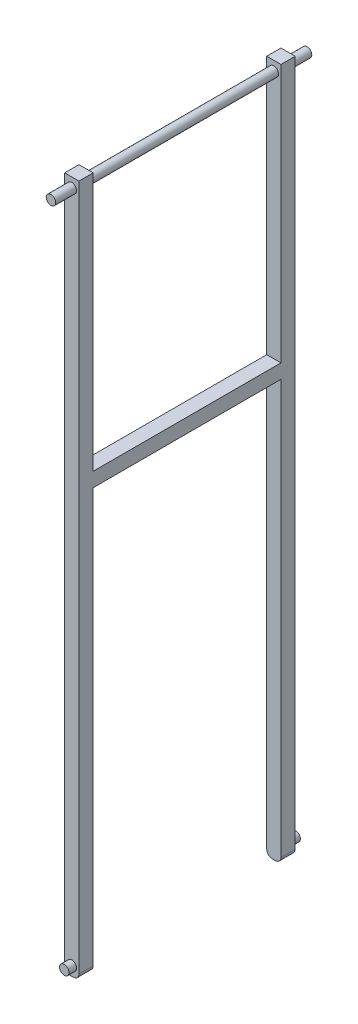
SolidWorks part; units mm, degrees
ref_plane "Front Plane" through (0, 0, 0) normal (0, 0, 1) x (1, 0, 0)
ref_plane "Top Plane" through (0, 0, 0) normal (0, 1, 0) x (1, 0, 0)
ref_plane "Right Plane" through (0, 0, 0) normal (1, 0, 0) x (0, 0, -1)
other "Configuration Table"
sketch "Sketch1" plane through (0, 0, 0) normal (0, 1, 0) x (1, 0, 0)
  line L1 (-7.5, 7.5) -> (7.5, 7.5)
  line L2 (-7.5, 7.5) -> (-7.5, -7.5)
  line L3 (-7.5, -7.5) -> (7.5, -7.5)
  line L4 (7.5, 7.5) -> (7.5, -7.5)
  line L5 (-7.5, 7.5) -> (7.5, -7.5) construction
  line L6 (-7.5, -7.5) -> (7.5, 7.5) construction
  point P0 (0, 0)
  dimension "D1" = 15
  dimension "D2" = 15
extrude "Boss-Extrude1" add sketch "Sketch1" along normal blind 730
sketch "Sketch2" plane through (0, 0, -7.5) normal (0, 0, -1) x (-1, 0, 0)
  circle A0 centre (0, 10) radius 5
  dimension "D1" = 10
  dimension "D2" = 10
extrude "Boss-Extrude2" add sketch "Sketch2" along normal blind 8
sketch "Sketch4" plane through (0, 0, 7.5) normal (0, 0, 1) x (1, 0, 0)
  line L0 (7.5, 730) -> (7.5, 0) construction
  line L1 (-7.5, 457.5) -> (7.5, 457.5)
  line L2 (-7.5, 457.5) -> (-7.5, 442.5)
  line L3 (-7.5, 442.5) -> (7.5, 442.5)
  line L4 (7.5, 457.5) -> (7.5, 442.5)
  line L5 (-7.5, 457.5) -> (7.5, 442.5) construction
  line L6 (-7.5, 442.5) -> (7.5, 457.5) construction
  line L7 (-7.5, 730) -> (7.5, 730) construction
  point P0 (0, 450)
  dimension "D1" = 15
  dimension "D2" = 15
  dimension "D3" = 450
  dimension "D4" = 280
extrude "Boss-Extrude3" add sketch "Sketch4" along normal blind 198
sketch "Sketch5" plane through (0, 0, 205.5) normal (0, 0, 1) x (1, 0, 0)
  line L0 (-7.5, 730) -> (-7.5, 457.5) construction
  line L1 (-7.5, 730) -> (7.5, 730)
  line L2 (-7.5, 730) -> (-7.5, 0)
  line L3 (-7.5, 0) -> (7.5, 0)
  line L4 (7.5, 730) -> (7.5, 0)
  line L5 (-7.5, 730) -> (7.5, 0) construction
  line L6 (-7.5, 0) -> (7.5, 730) construction
  point P0 (0, 365)
extrude "Boss-Extrude4" add sketch "Sketch5" along normal blind 15
sketch "Sketch6" plane through (0, 0, 220.5) normal (0, 0, 1) x (1, 0, 0)
  circle A0 centre (0, 10) radius 5
  dimension "D1" = 10
  dimension "D2" = 10
extrude "Boss-Extrude5" add sketch "Sketch6" along normal blind 8
fillet "Fillet1" radius 6 4 edges at (-7.5, 0, 213) (7.5, 0, 213) (-7.5, 0, 0) (7.5, 0, 0)
sketch "Sketch7" plane through (0, 0, -7.5) normal (0, 0, -1) x (-1, 0, 0)
  line L0 (0, 730) -> (0, 720) construction
  line L1 (-7.5, 730) -> (7.5, 730) construction
  circle A0 centre (0, 720) radius 5
  dimension "D1" = 10
  dimension "D2" = 10
extrude "Boss-Extrude6" add sketch "Sketch7" against normal blind 250 and the other way blind 20
